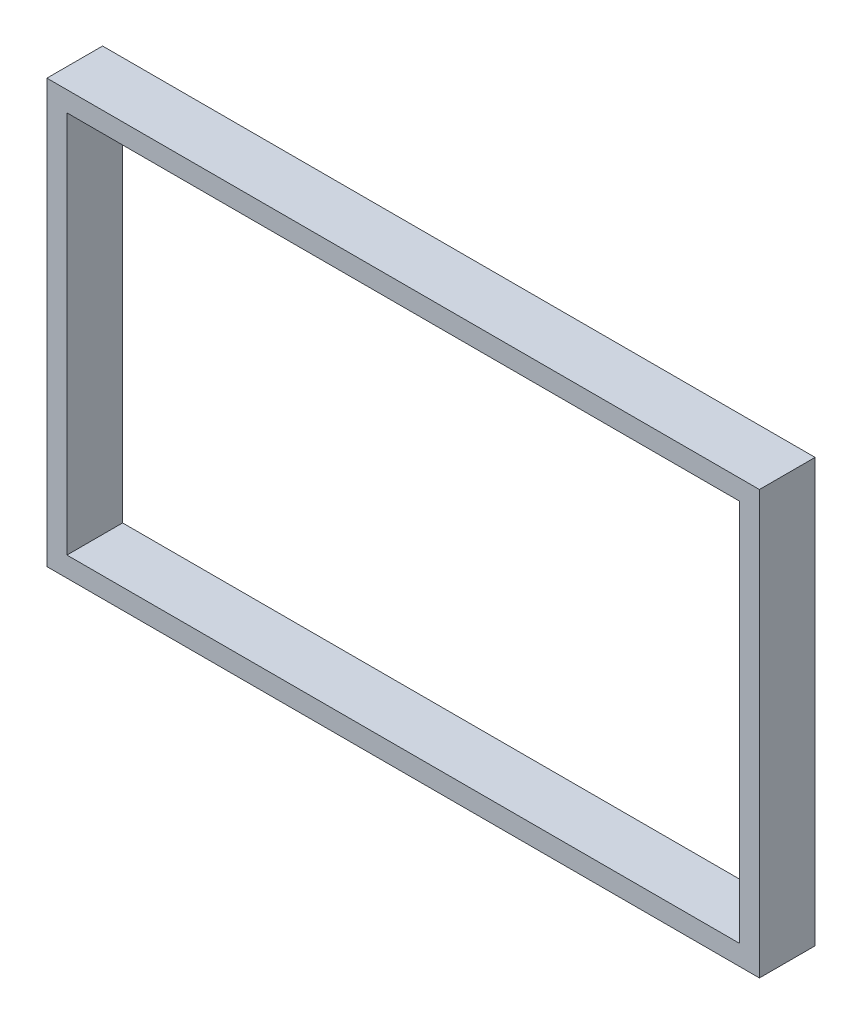
SolidWorks part; units mm, degrees
ref_plane "前视基准面" through (0, 0, 0) normal (0, 0, 1) x (1, 0, 0)
ref_plane "上视基准面" through (0, 0, 0) normal (0, 1, 0) x (1, 0, 0)
ref_plane "右视基准面" through (0, 0, 0) normal (1, 0, 0) x (0, 0, -1)
other "Configuration Table"
sketch "草图1" plane through (0, 0, 0) normal (0, 0, 1) x (1, 0, 0)
  line L0 (-32, -19) -> (32, -19)
  line L1 (32, -19) -> (32, 19)
  line L2 (32, 19) -> (-32, 19)
  line L3 (-32, 19) -> (-32, -19)
  line L4 (-30.2, -17.2) -> (30.2, -17.2)
  line L5 (30.2, -17.2) -> (30.2, 17.2)
  line L6 (30.2, 17.2) -> (-30.2, 17.2)
  line L7 (-30.2, 17.2) -> (-30.2, -17.2)
  point P0 (0, 0)
  dimension "D1" = 1.8
  dimension "D2" = 32
  dimension "D3" = 62.2
  dimension "D4" = 64
  dimension "D5" = 1.8
  dimension "D6" = 19
  dimension "D7" = 36.2
  dimension "D8" = 38
extrude "凸台-拉伸1" add sketch "草图1" against normal mid plane 5
